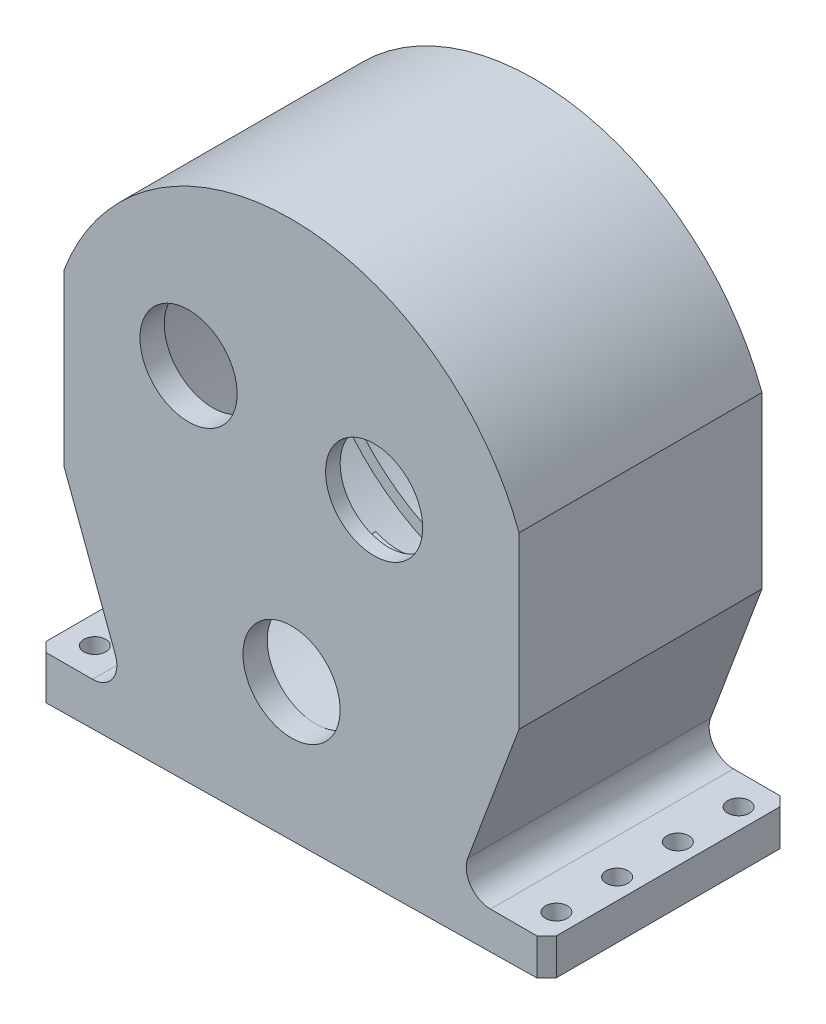
SolidWorks part; units mm, degrees
material "AISI 1045 Steel, Cold Drawn"
ref_plane "Front Plane" through (0, 0, 0) normal (0, 0, 1) x (1, 0, 0)
ref_plane "Top Plane" through (0, 0, 0) normal (0, 1, 0) x (1, 0, 0)
ref_plane "Right Plane" through (0, 0, 0) normal (1, 0, 0) x (0, 0, -1)
other "Configuration Table"
sketch "Sketch1" plane through (0, 0, 0) normal (0, 0, 1) x (1, 0, 0)
  circle A0 centre (0, 0) radius 50
  dimension "D1" = 100
extrude "Boss-Extrude1" add sketch "Sketch1" along normal blind 50
sketch "Sketch2" plane through (0, 0, 0) normal (0, 0, -1) x (-1, 0, 0)
  circle A0 centre (0, 0) radius 42.5
  dimension "D1" = 85
extrude "Cut-Extrude1" cut sketch "Sketch2" against normal blind 45
sketch "Sketch3" plane through (0, 0, 45) normal (0, 0, -1) x (-1, 0, 0)
  circle A0 centre (0, 0) radius 12.5
  dimension "D1" = 25
extrude "Cut-Extrude2" cut sketch "Sketch3" against normal blind 2
sketch "Sketch4" plane through (0, 0, 45) normal (0, 0, -1) x (-1, 0, 0)
  line L0 (-58.4465, 0) -> (76.9948, 0) construction
  line L1 (0, 55.8679) -> (0, -63.2033) construction
  circle A0 centre (0, 0) radius 19 construction
  circle A1 centre (0, 0) radius 25 construction
  circle A2 centre (0, 0) radius 32.5 construction
  circle A4 centre (-17, 8.4853) radius 10
  circle A5 centre (21.2, 13.2499) radius 10
  circle A6 centre (0, -32.5) radius 10
  dimension "D1" = 38
  dimension "D2" = 50
  dimension "D3" = 65
  dimension "D4" = 20
  dimension "D5" = 20
  dimension "D6" = 20
  dimension "D7" = 17
  dimension "D8" = 21.2
extrude "Cut-Extrude3" cut sketch "Sketch4" against normal through all
sketch "Sketch5" plane through (0, 0, 0) normal (0, 0, -1) x (-1, 0, 0)
  line L0 (-46.8336, -17.5104) -> (-33.7476, -52.5104)
  line L1 (46.8336, -17.5104) -> (33.7476, -52.5104)
  line L2 (86.1882, -52.5104) -> (33.7476, -52.5104) construction
  line L3 (-52.5, -52.5104) -> (-33.7476, -52.5104)
  line L4 (52.5, -52.5104) -> (52.5, -61.5104)
  line L5 (52.5, -61.5104) -> (-52.5, -59.9896)
  line L6 (-52.5, -59.9896) -> (-52.5, -52.5104)
  line L7 (0, -67.3761) -> (0, 67.3761) construction
  line L8 (-33.7476, -52.5104) -> (-52.5, -52.5104) construction
  line L9 (33.7476, -52.5104) -> (52.5, -52.5104)
  circle A0 centre (0, 0) radius 50 construction
  arc A1 (-46.8336, -17.5104) -> (46.8336, -17.5104) centre (0, 0) ccw
  point P10 (16.8441, -52.5104)
  point P17 (0, 0)
  dimension "D1" = 69.5
  dimension "D2" = 69.5
  dimension "D3" = 35
  dimension "D4" = 9
  dimension "D5" = 105
extrude "Boss-Extrude2" add sketch "Sketch5" against normal blind 50
sketch "Sketch6" plane through (0, 0, 0) normal (0, 0, -1) x (-1, 0, 0)
  line L0 (-46.8336, -17.5104) -> (-46.8336, 17.5104)
  line L1 (46.8336, -17.5104) -> (46.8336, 17.5104)
  arc A0 (46.8336, -17.5104) -> (-46.8336, -17.5104) centre (0, 0) ccw construction
  arc A1 (46.8336, -17.5104) -> (46.8336, 17.5104) centre (0, 0) ccw
  arc A2 (-46.8336, 17.5104) -> (-46.8336, -17.5104) centre (0, 0) ccw
extrude "Cut-Extrude4" cut sketch "Sketch6" against normal through all
sketch "Sketch7" plane through (0.8797, -60.7372, 0) normal (0.0145, -0.9999, 0) x (0.9999, 0.0145, 0)
  line L0 (0, -21.8323) -> (0, 62.7533) construction
  line L1 (-62.5769, 25) -> (63.2424, 25) construction
  line L2 (51.6257, 50) -> (-53.3853, 50) construction
  line L3 (51.6257, 0) -> (-53.3853, 0) construction
  line L4 (51.6257, 0) -> (-53.3853, 0) construction
  line L5 (51.6257, 50) -> (-53.3853, 50) construction
  circle A0 centre (-47.5, 43.75) radius 2.25
  circle A1 centre (-47.5, 31.25) radius 2.25
  circle A2 centre (47.5, 31.25) radius 2.25
  circle A3 centre (47.5, 43.75) radius 2.25
  circle A4 centre (47.5, 18.75) radius 2.25
  circle A5 centre (47.5, 6.25) radius 2.25
  circle A6 centre (-47.5, 18.75) radius 2.25
  circle A7 centre (-47.5, 6.25) radius 2.25
  point P4 (0, 20.4605)
  dimension "D1" = 4.5
  dimension "D2" = 4.5
  dimension "D3" = 47.5
  dimension "D4" = 47.5
  dimension "D5" = 6.25
  dimension "D6" = 18.75
extrude "Cut-Extrude5" cut sketch "Sketch7" against normal blind 20
fillet "Fillet1" radius 5 1 edges at (33.7476, -52.5104, 25)
fillet "Fillet2" radius 5 1 edges at (-33.7476, -52.5104, 25)
chamfer "Chamfer1" distance 2 angle 45 4 edges at (52.5, -56.25, 50) (-52.5, -57.0104, 50) (-52.5, -57.0104, 0) (52.5, -56.25, 0)
sketch "Sketch8" plane through (0, 0, 47) normal (0, 0, -1) x (-1, 0, 0)
  circle A0 centre (0, 0) radius 4
  dimension "D1" = 8
extrude "Cut-Extrude6" cut sketch "Sketch8" against normal blind 1
sketch "Sketch9" plane through (0, 0, 45) normal (0, 0, -1) x (-1, 0, 0)
  circle A0 centre (-17, 8.4853) radius 11.5
  dimension "D1" = 23
extrude "Cut-Extrude8" cut sketch "Sketch9" against normal blind 2
sketch "Sketch10" plane through (0, 0, 0) normal (0, 0, -1) x (-1, 0, 0)
  circle A0 centre (0, 0) radius 40
  circle A1 centre (0, 0) radius 42.5
  dimension "D1" = 80
extrude "Boss-Extrude3" add sketch "Sketch10" against normal blind 5
sketch "Sketch11" plane through (0, 0, 0) normal (0, 0, -1) x (-1, 0, 0)
  line L0 (66.8973, 0) -> (-66.8973, 0) construction
  circle A0 centre (0, 46) radius 2
  circle A1 centre (23, 39.8372) radius 2
  circle A2 centre (39.8372, 23) radius 2
  circle A3 centre (-23, 39.8372) radius 2
  circle A4 centre (-39.8372, 23) radius 2
  circle A5 centre (39.8372, -23) radius 2
  circle A6 centre (23, -39.8372) radius 2
  circle A7 centre (0, -46) radius 2
  circle A8 centre (-23, -39.8372) radius 2
  circle A9 centre (-39.8372, -23) radius 2
  point P9 (0, 0)
  point P14 (0, 0)
  point P17 (0, 0)
  dimension "D1" = 4
  dimension "D2" = 46
  dimension "D3" = 3
  dimension "D4" = 3
extrude "Cut-Extrude9" cut sketch "Sketch11" against normal blind 8
